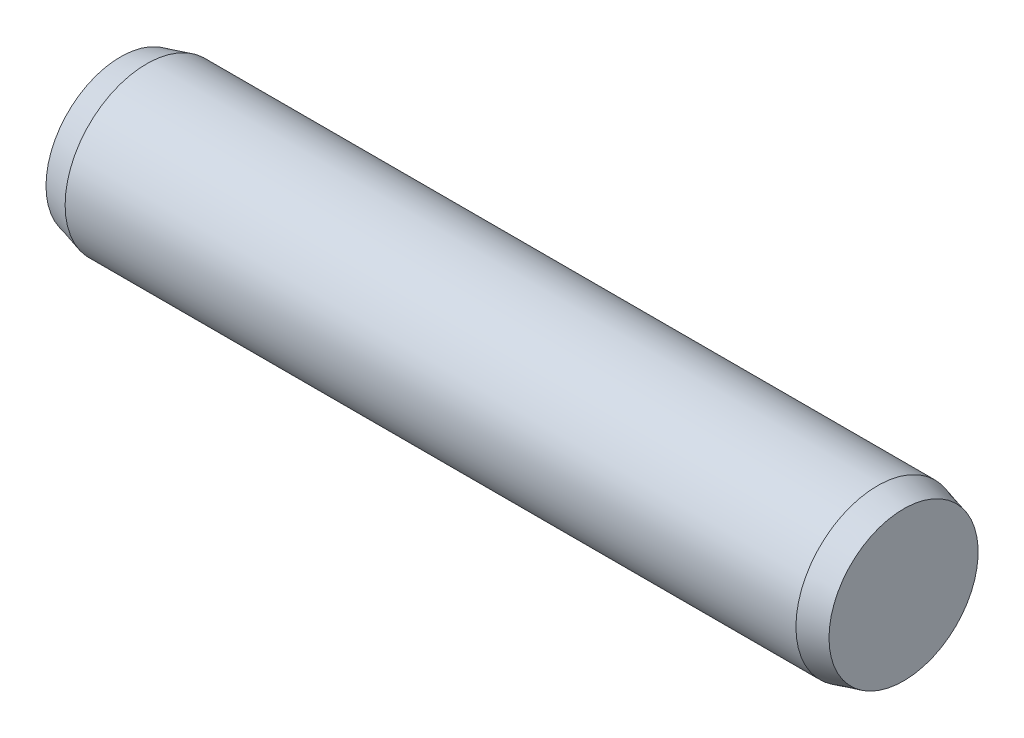
from build123d import *


with BuildPart() as part:
    # Sketch1 → Base-Revolve (revolve)
    with BuildSketch(Plane.XY, mode=Mode.PRIVATE) as base_revolve_sk:
        Polygon((-1.4, 0), (10.6, 0), (10.6, 1.142820323), (10.2, 1.25), (-1, 1.25), (-1.4, 1.142820323), align=None)
    revolve(base_revolve_sk.sketch.rotate(Axis((0, 0, 0), (1, 0, 0)), 90), axis=Axis((0, 0, 0), (1, 0, 0)))


solid = part.part
